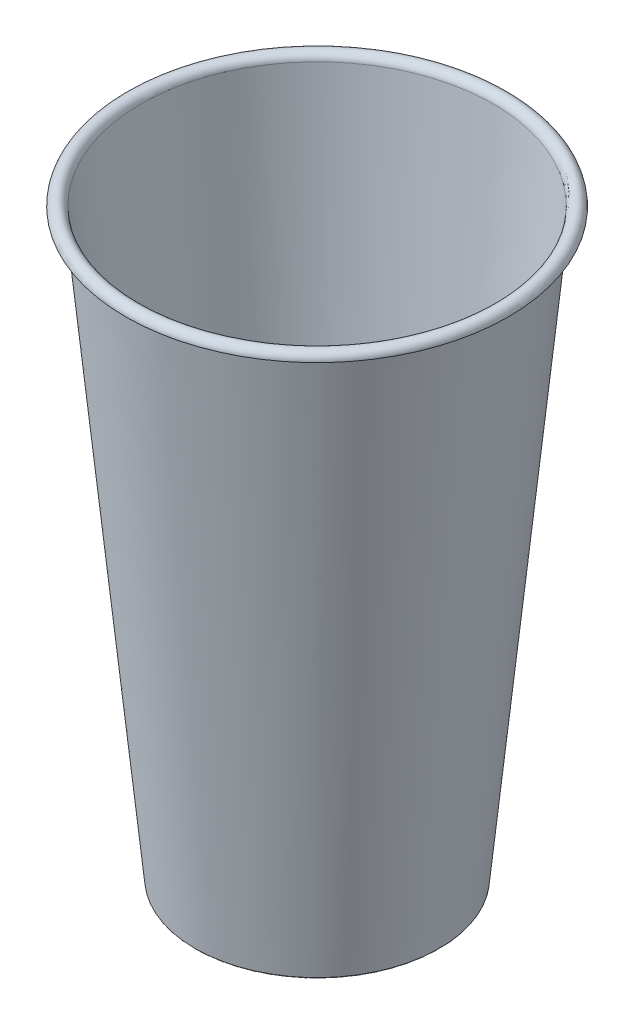
from build123d import *


with BuildPart() as part:
    # 草图1 → 旋转1 (revolve)
    with BuildSketch(Plane.XY, mode=Mode.PRIVATE) as revolve_1_sk:
        with BuildLine():
            Line((0, 0), (28.15, 0))
            Line((28.15, 0), (41, 131.6))
            ThreePointArc((41, 131.6), (42.826851784, 133.177859086), (44.491716565, 131.429931171))
            Line((44.491716565, 131.429931171), (43.891716565, 131.429931171))
            ThreePointArc((43.891716565, 131.429931171), (42.797662566, 132.578569515), (41.597159965, 131.541690687))
            Line((41.597159965, 131.541690687), (28.374048388, -3.879436438))
            ThreePointArc((28.374048388, -3.879436438), (28.309369008, -4.008133871), (28.174995066, -4.06))
            Line((28.174995066, -4.06), (27.974043886, -4.06))
            ThreePointArc((27.974043886, -4.06), (27.825910015, -3.994373942), (27.774990564, -3.840563562))
            Line((27.774990564, -3.840563562), (28.091413374, -0.6))
            Line((28.091413374, -0.6), (0, -0.6))
            Line((0, -0.6), (0, 0))
        make_face()
    revolve(revolve_1_sk.sketch.rotate(Axis((0, 0, 0), (0, -1, 0)), 90), axis=Axis((0, 0, 0), (0, -1, 0)))


solid = part.part
